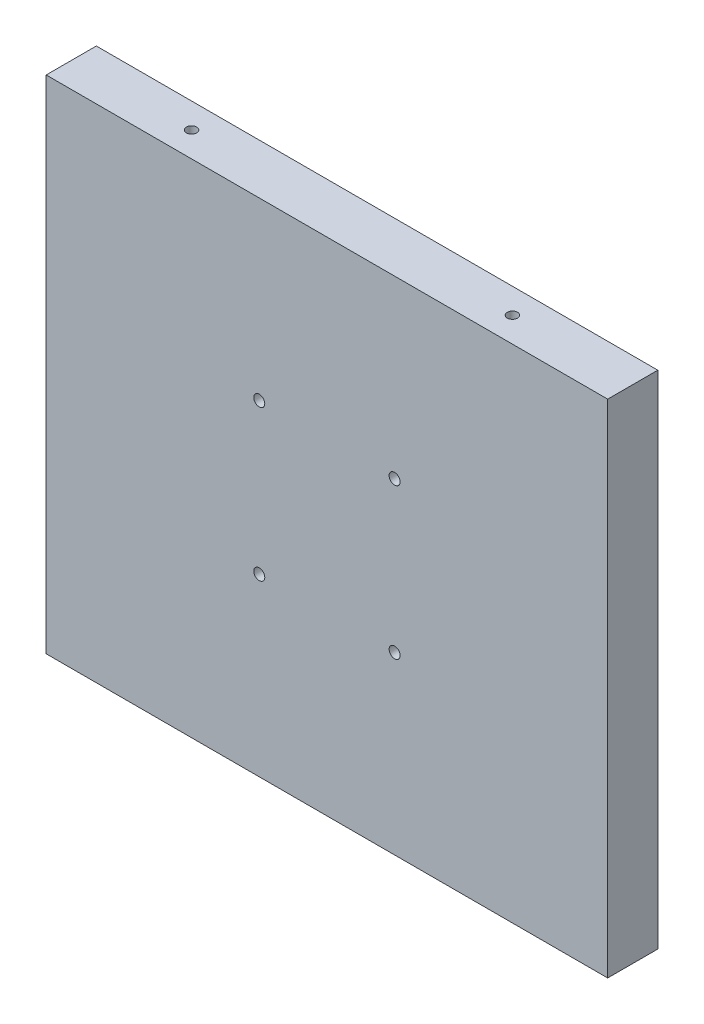
SolidWorks part; units mm, degrees
material "1023 碳钢板 (SS)"
ref_plane "前视基准面" through (0, 0, 0) normal (0, 0, 1) x (1, 0, 0)
ref_plane "上视基准面" through (0, 0, 0) normal (0, 1, 0) x (1, 0, 0)
ref_plane "右视基准面" through (0, 0, 0) normal (1, 0, 0) x (0, 0, -1)
sketch "草图1" plane through (0, 0, 0) normal (0, 0, 1) x (1, 0, 0)
  line L1 (280, 250) -> (-280, 250)
  line L2 (280, 250) -> (280, -250)
  line L3 (280, -250) -> (-280, -250)
  line L4 (-280, 250) -> (-280, -250)
  line L5 (280, 250) -> (-280, -250) construction
  line L6 (280, -250) -> (-280, 250) construction
  point P0 (0, 0)
  dimension "D1" = 560
  dimension "D2" = 500
extrude "凸台-拉伸1" add sketch "草图1" along normal blind 50
sketch "草图2" plane through (0, 250, 0) normal (0, 1, 0) x (1, 0, 0)
  line L0 (280, 0) -> (-280, 0) construction
  circle A0 centre (-160, -25) radius 17.1374
  circle A1 centre (160, -25) radius 12.7027
  point P5 (0, 0)
  point P8 (0, 0)
  dimension "D1" = 320
  dimension "D2" = 160
  dimension "D3" = 25
hole_wizard "M12 螺纹孔1" positions "草图3" profile "草图4" tap size "M12" standard "ISO"
sketch "草图3" plane through (0, 250, 0) normal (0, 1, 0) x (1, 0, 0)
  point P0 (-160, -25)
  point P3 (160, -25)
sketch "草图4" plane through (-160, 250, 25) normal (1, 0, 0) x (0, 0, 1)
  line L0 (0, 0) -> (0, 32.3144)
  line L1 (0, 32.3144) -> (5.1, 29.25)
  line L2 (5.1, 29.25) -> (5.1, 0)
  line L5 (5.1, 0) -> (0, 0)
  line L10 (0, 32.3144) -> (-5.1, 29.25) construction
  line L11 (0, -6.35) -> (0, 107.95) construction
  dimension "螺纹孔钻头直径" = 10.2
  dimension "螺纹孔钻头深度" = 29.25
  dimension "导头角度" = 118
cosmetic thread "孔螺蚊线1" parameters "D1"=24, "D2"=12
cosmetic thread "孔螺蚊线2" parameters "D1"=24, "D2"=12
sketch "草图5" plane through (0, 0, 50) normal (0, 0, 1) x (1, 0, 0)
  circle A0 centre (-67.5, 75) radius 5.5
  circle A1 centre (67.5, 75) radius 5.5
  circle A2 centre (67.5, -75) radius 5.5
  circle A3 centre (-67.5, -75) radius 5.5
  point P8 (0, 0)
  point P9 (0, 0)
  point P10 (0, 0)
  point P11 (0, 0)
  dimension "D2" = 135
  dimension "D5" = 11
  dimension "D1" = 150
  dimension "D3" = 67.5
  dimension "D4" = 75
extrude "切除-拉伸1" cut sketch "草图5" against normal blind 50
